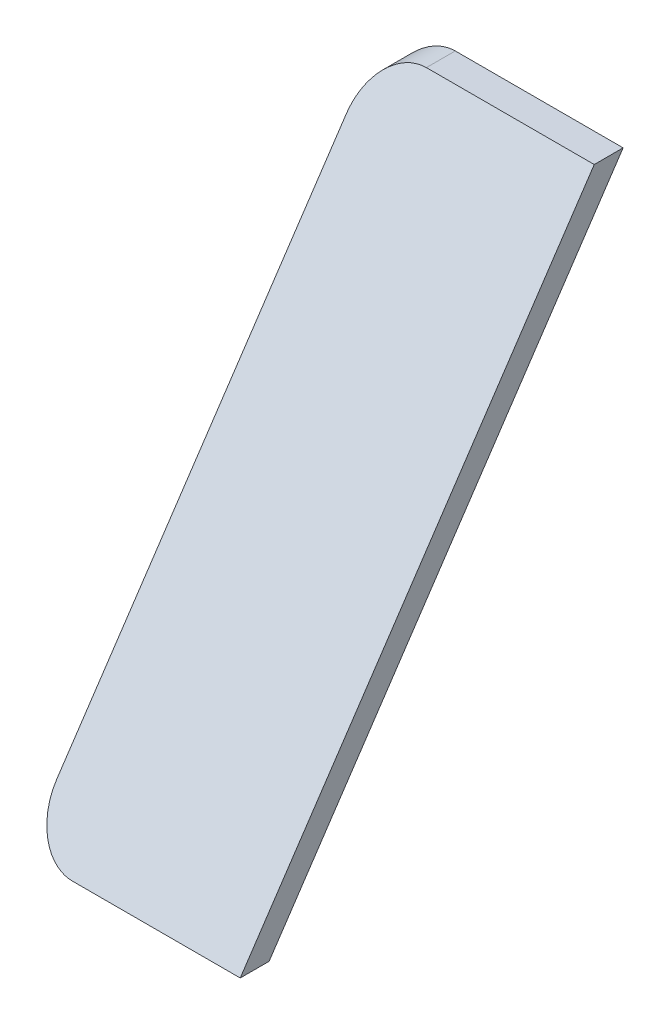
SolidWorks part; units mm, degrees
ref_plane "前视基准面" through (0, 0, 0) normal (0, 0, 1) x (1, 0, 0)
ref_plane "上视基准面" through (0, 0, 0) normal (0, 1, 0) x (1, 0, 0)
ref_plane "右视基准面" through (0, 0, 0) normal (1, 0, 0) x (0, 0, -1)
sketch "草图1" plane through (0, 0, 0) normal (0, 0, 1) x (1, 0, 0)
  line L0 (-679.8213, 67.7) -> (-679.8213, -42.3)
  line L1 (-679.8213, -42.3) -> (-679.5468, -41.7323)
  line L7 (-679.8213, 67.7) -> (-714.8213, 67.7)
  line L33 (-679.8213, -42.3) -> (-714.8213, -42.3)
  line L34 (-724.8213, -32.3) -> (-724.8213, 57.7)
  arc A12 (-724.8213, -32.3) -> (-714.8213, -42.3) centre (-714.8213, -32.3) ccw
  arc A13 (-714.8213, 67.7) -> (-724.8213, 57.7) centre (-714.8213, 57.7) ccw
extrude "凸台-拉伸2" add sketch "草图1" along normal blind 100 contours L33 A12 L34 A13 L7 L0
sketch "草图3" plane through (-679.8213, 0, 0) normal (1, 0, 0) x (0, 0, -1)
  line L0 (0, -42.3) -> (-80, -42.3)
  line L1 (-100, -42.3) -> (0, -42.3) construction
  line L6 (-100, 67.7) -> (0, 67.7) construction
  line L8 (-6.1825, 67.7) -> (-80, -42.3)
  line L12 (-10.3343, 70.4861) -> (-84.1518, -39.5139)
  line L13 (-10.3343, 70.4861) -> (-86.0215, -42.3)
  line L14 (-86.0215, -42.3) -> (-80, -42.3)
  line L15 (-6.1825, 67.7) -> (-12.204, 67.7)
  dimension "D1" = 5
extrude "切除-拉伸5" cut sketch "草图3" against normal blind 100 flip side to cut
